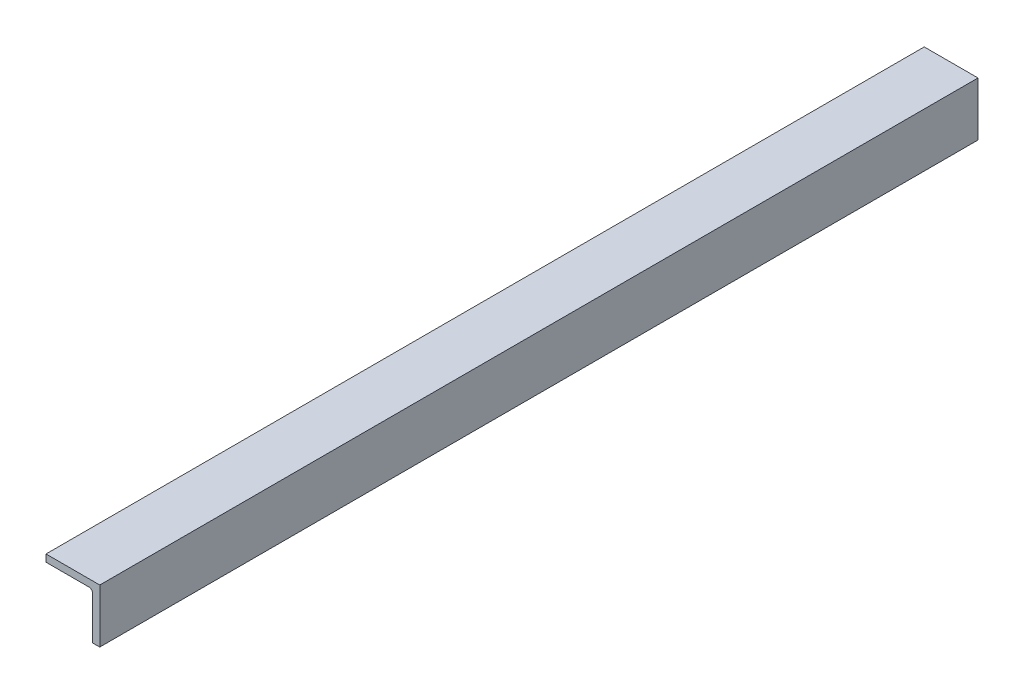
SolidWorks part; units mm, degrees
material "1023 碳钢板 (SS)"
ref_plane "Front Plane" through (0, 0, 0) normal (0, 0, 1) x (1, 0, 0)
ref_plane "Top Plane" through (0, 0, 0) normal (0, 1, 0) x (1, 0, 0)
ref_plane "Right Plane" through (0, 0, 0) normal (1, 0, 0) x (0, 0, -1)
sketch "Sketch1" plane through (0, 0, 0) normal (0, 0, 1) x (1, 0, 0)
  line L0 (0, 0) -> (30, 0)
  line L1 (30, 0) -> (30, -30)
  line L2 (0, -4) -> (24, -4)
  line L3 (26, -6) -> (26, -30)
  line L4 (0, 0) -> (0, -4)
  line L5 (30, -30) -> (26, -30)
  line L6 (0, -4) -> (26, -4) construction
  line L7 (26, -4) -> (26, -30) construction
  arc A0 (24, -4) -> (26, -6) centre (24, -6) cw
  dimension "D4" = 2
  dimension "D1" = 30
  dimension "D2" = 30
  dimension "D3" = 4
extrude "Boss-Extrude1" add sketch "Sketch1" along normal blind 490 contours L5 L3 A0 L2 L4 L0 L1
